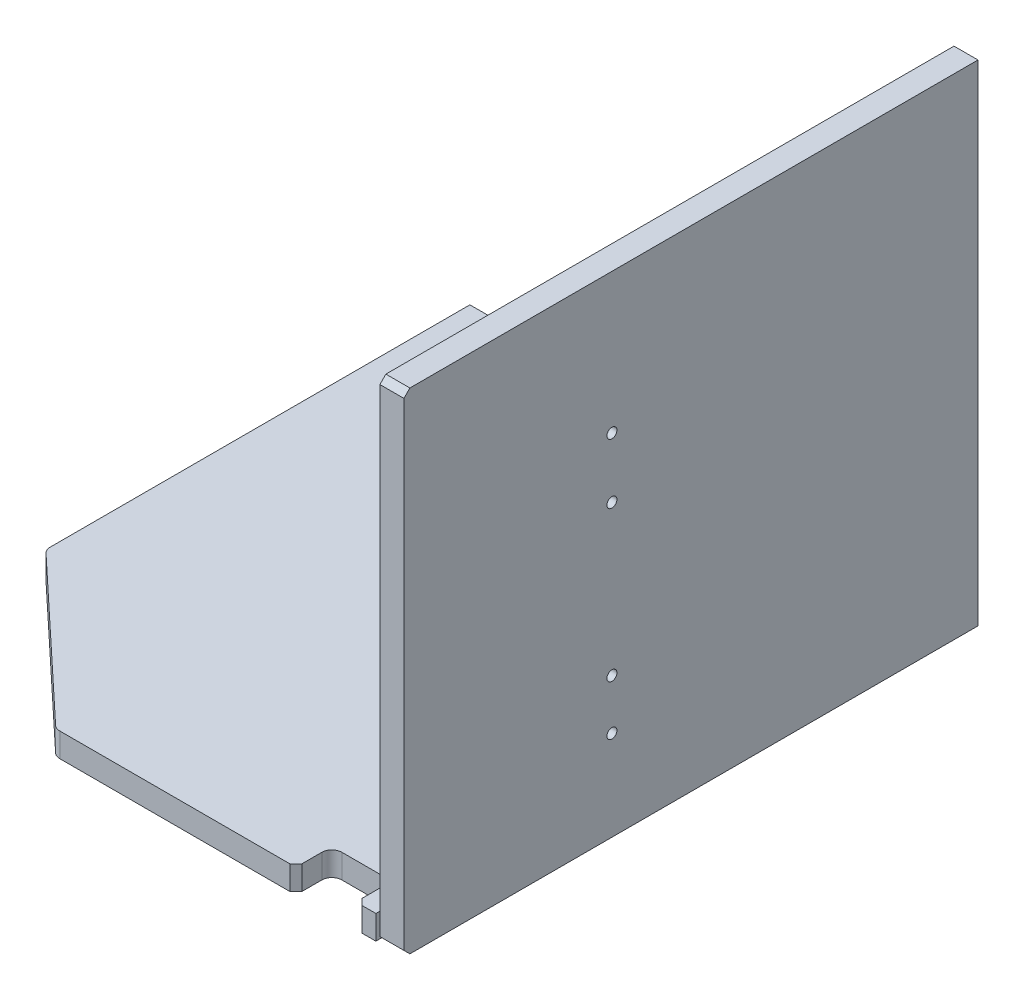
from build123d import *

# Parameters (mm, degrees)
SKETCH1_W                  = 12
SKETCH1_H                  = 245
BOSS_EXTRUDE1_DEPTH        = 287
SKETCH1_W_2                = 240
SKETCH1_H_2                = 12
BOSS_EXTRUDE1_2_DEPTH      = 287
SKETCH3_W                  = 30
SKETCH3_H                  = 18
CUT_EXTRUDE1_DEPTH         = 403.484782321
M5_TAPPED_HOLE1_AT_2_COUNT = 2
M5_TAPPED_HOLE1_AT_2_PITCH = 90
M5_TAPPED_HOLE1_AT_3_COUNT = 2
M5_TAPPED_HOLE1_AT_3_PITCH = 180
M5_TAPPED_HOLE1_AT_4_COUNT = 2
M5_TAPPED_HOLE1_AT_4_PITCH = 215.896387186
M5_TAPPED_HOLE1_AT_5_COUNT = 2
M5_TAPPED_HOLE1_AT_5_PITCH = 242.953184791
M5_TAPPED_HOLE1_AT_6_COUNT = 2
M5_TAPPED_HOLE1_AT_6_PITCH = 289.570803086
CHAMFER1_SIZE              = 3
FILLET1_R                  = 5
CHAMFER2_SIZE              = 3
M6_TAPPED_HOLE1_AT_2_COUNT = 2
M6_TAPPED_HOLE1_AT_2_PITCH = 130
M6_TAPPED_HOLE2_AT_2_COUNT = 2
M6_TAPPED_HOLE2_AT_2_PITCH = 75
CUT_EXTRUDE3_DEPTH         = 396.29482668
FILLET3_R                  = 5


with BuildPart() as part:
    # Sketch1 → Boss-Extrude1 (new body)
    with BuildSketch(Plane.XY):
        with Locations((134, -17.5)):
            Rectangle(SKETCH1_W, SKETCH1_H)
    extrude(amount=BOSS_EXTRUDE1_DEPTH)

    # Sketch5 → M5 Tapped Hole1 (revolve, cut)
    with BuildSketch(Plane(origin=(134, 72.5, 0), x_dir=(0, 1, 0), z_dir=(1, 0, 0))):
        Polygon((0, 0), (0, 15.2618073), (2.1, 14), (2.1, 0), align=None)
    m5_tapped_hole1 = revolve(axis=Axis((134, 72.5, -6.35), (0, 0, 1)), mode=Mode.SUBTRACT)

    # M5 Tapped Hole1 at 2: M5 Tapped Hole1 ×2
    with Locations(*[(0, -i * M5_TAPPED_HOLE1_AT_2_PITCH, 0) for i in range(1, M5_TAPPED_HOLE1_AT_2_COUNT)]):
        add(m5_tapped_hole1, mode=Mode.SUBTRACT)

    # M5 Tapped Hole1 at 3: M5 Tapped Hole1 ×2
    with Locations(*[(0, -i * M5_TAPPED_HOLE1_AT_3_PITCH, 0) for i in range(1, M5_TAPPED_HOLE1_AT_3_COUNT)]):
        add(m5_tapped_hole1, mode=Mode.SUBTRACT)

    # Chamfer2
    chamfer2_edges = [part.edges().sort_by_distance(p)[0] for p in [
        (134, -140, 287),
        (134, 105, 287),
    ]]
    chamfer(chamfer2_edges, length=CHAMFER2_SIZE)

    # Sketch8 → M6 Tapped Hole1 (revolve, cut)
    with BuildSketch(Plane(origin=(140, 35, 183), x_dir=(0, 0, -1), z_dir=(0, 1, 0))):
        Polygon((0, 0), (0, 18.502151548), (2.5, 17), (2.5, 0), align=None)
    m6_tapped_hole1 = revolve(axis=Axis((146.35, 35, 183), (-1, 0, 0)), mode=Mode.SUBTRACT)

    # M6 Tapped Hole1 at 2: M6 Tapped Hole1 ×2
    with Locations(*[(0, -i * M6_TAPPED_HOLE1_AT_2_PITCH, 0) for i in range(1, M6_TAPPED_HOLE1_AT_2_COUNT)]):
        add(m6_tapped_hole1, mode=Mode.SUBTRACT)

    # Sketch10 → M6 Tapped Hole2 (revolve, cut)
    with BuildSketch(Plane(origin=(140, -70, 183), x_dir=(0, 0, -1), z_dir=(0, 1, 0))):
        Polygon((0, 0), (0, 18.502151548), (2.5, 17), (2.5, 0), align=None)
    m6_tapped_hole2 = revolve(axis=Axis((146.35, -70, 183), (-1, 0, 0)), mode=Mode.SUBTRACT)

    # M6 Tapped Hole2 at 2: M6 Tapped Hole2 ×2
    with Locations(*[(0, i * M6_TAPPED_HOLE2_AT_2_PITCH, 0) for i in range(1, M6_TAPPED_HOLE2_AT_2_COUNT)]):
        add(m6_tapped_hole2, mode=Mode.SUBTRACT)


with BuildPart() as body_2:
    # Sketch1 → Boss-Extrude1 2 (new body)
    with BuildSketch(Plane.XY):
        with Locations((6, -134)):
            Rectangle(SKETCH1_W_2, SKETCH1_H_2)
    extrude(amount=BOSS_EXTRUDE1_2_DEPTH)

    # Sketch3 → Cut-Extrude1 (cut, through all)
    with BuildSketch(Plane.XZ.offset(140)):
        with Locations((101, 278)):
            Rectangle(SKETCH3_W, SKETCH3_H)
    extrude(amount=-CUT_EXTRUDE1_DEPTH, mode=Mode.SUBTRACT)

    # M5 Tapped Hole1 at 4: M5 Tapped Hole1 ×2
    with Locations(*[Vector(-0.2918066430898717, -0.9564773301279128, 0) * (i * M5_TAPPED_HOLE1_AT_4_PITCH) for i in range(1, M5_TAPPED_HOLE1_AT_4_COUNT)]):
        add(m5_tapped_hole1, mode=Mode.SUBTRACT)

    # M5 Tapped Hole1 at 5: M5 Tapped Hole1 ×2
    with Locations(*[Vector(-0.526850471666832, -0.8499579874937565, 0) * (i * M5_TAPPED_HOLE1_AT_5_PITCH) for i in range(1, M5_TAPPED_HOLE1_AT_5_COUNT)]):
        add(m5_tapped_hole1, mode=Mode.SUBTRACT)

    # M5 Tapped Hole1 at 6: M5 Tapped Hole1 ×2
    with Locations(*[Vector(-0.7010375280810152, -0.7131243820134465, 0) * (i * M5_TAPPED_HOLE1_AT_6_PITCH) for i in range(1, M5_TAPPED_HOLE1_AT_6_COUNT)]):
        add(m5_tapped_hole1, mode=Mode.SUBTRACT)

    # Chamfer1
    chamfer1_edges = [body_2.edges().sort_by_distance(p)[0] for p in [
        (116, -134, 287),
        (86, -134, 287),
        (-114, -134, 287),
    ]]
    chamfer(chamfer1_edges, length=CHAMFER1_SIZE)

    # Fillet1
    fillet1_edges = [body_2.edges().sort_by_distance(p)[0] for p in [
        (86, -134, 269),
        (116, -134, 269),
    ]]
    fillet(fillet1_edges, radius=FILLET1_R)

    # Sketch11 → Cut-Extrude3 (cut, through all)
    with BuildSketch(Plane(origin=(0, -128, 0), x_dir=(1, 0, 0), z_dir=(0, 1, 0))):
        Polygon((-34, -287), (-114, -212), (-114, -287), align=None)
    extrude(amount=-CUT_EXTRUDE3_DEPTH, mode=Mode.SUBTRACT)

    # Fillet3
    fillet3_edges = [body_2.edges().sort_by_distance(p)[0] for p in [
        (-34, -134, 287),
        (-114, -134, 212),
    ]]
    fillet(fillet3_edges, radius=FILLET3_R)


solid = Compound([part.part, body_2.part])
